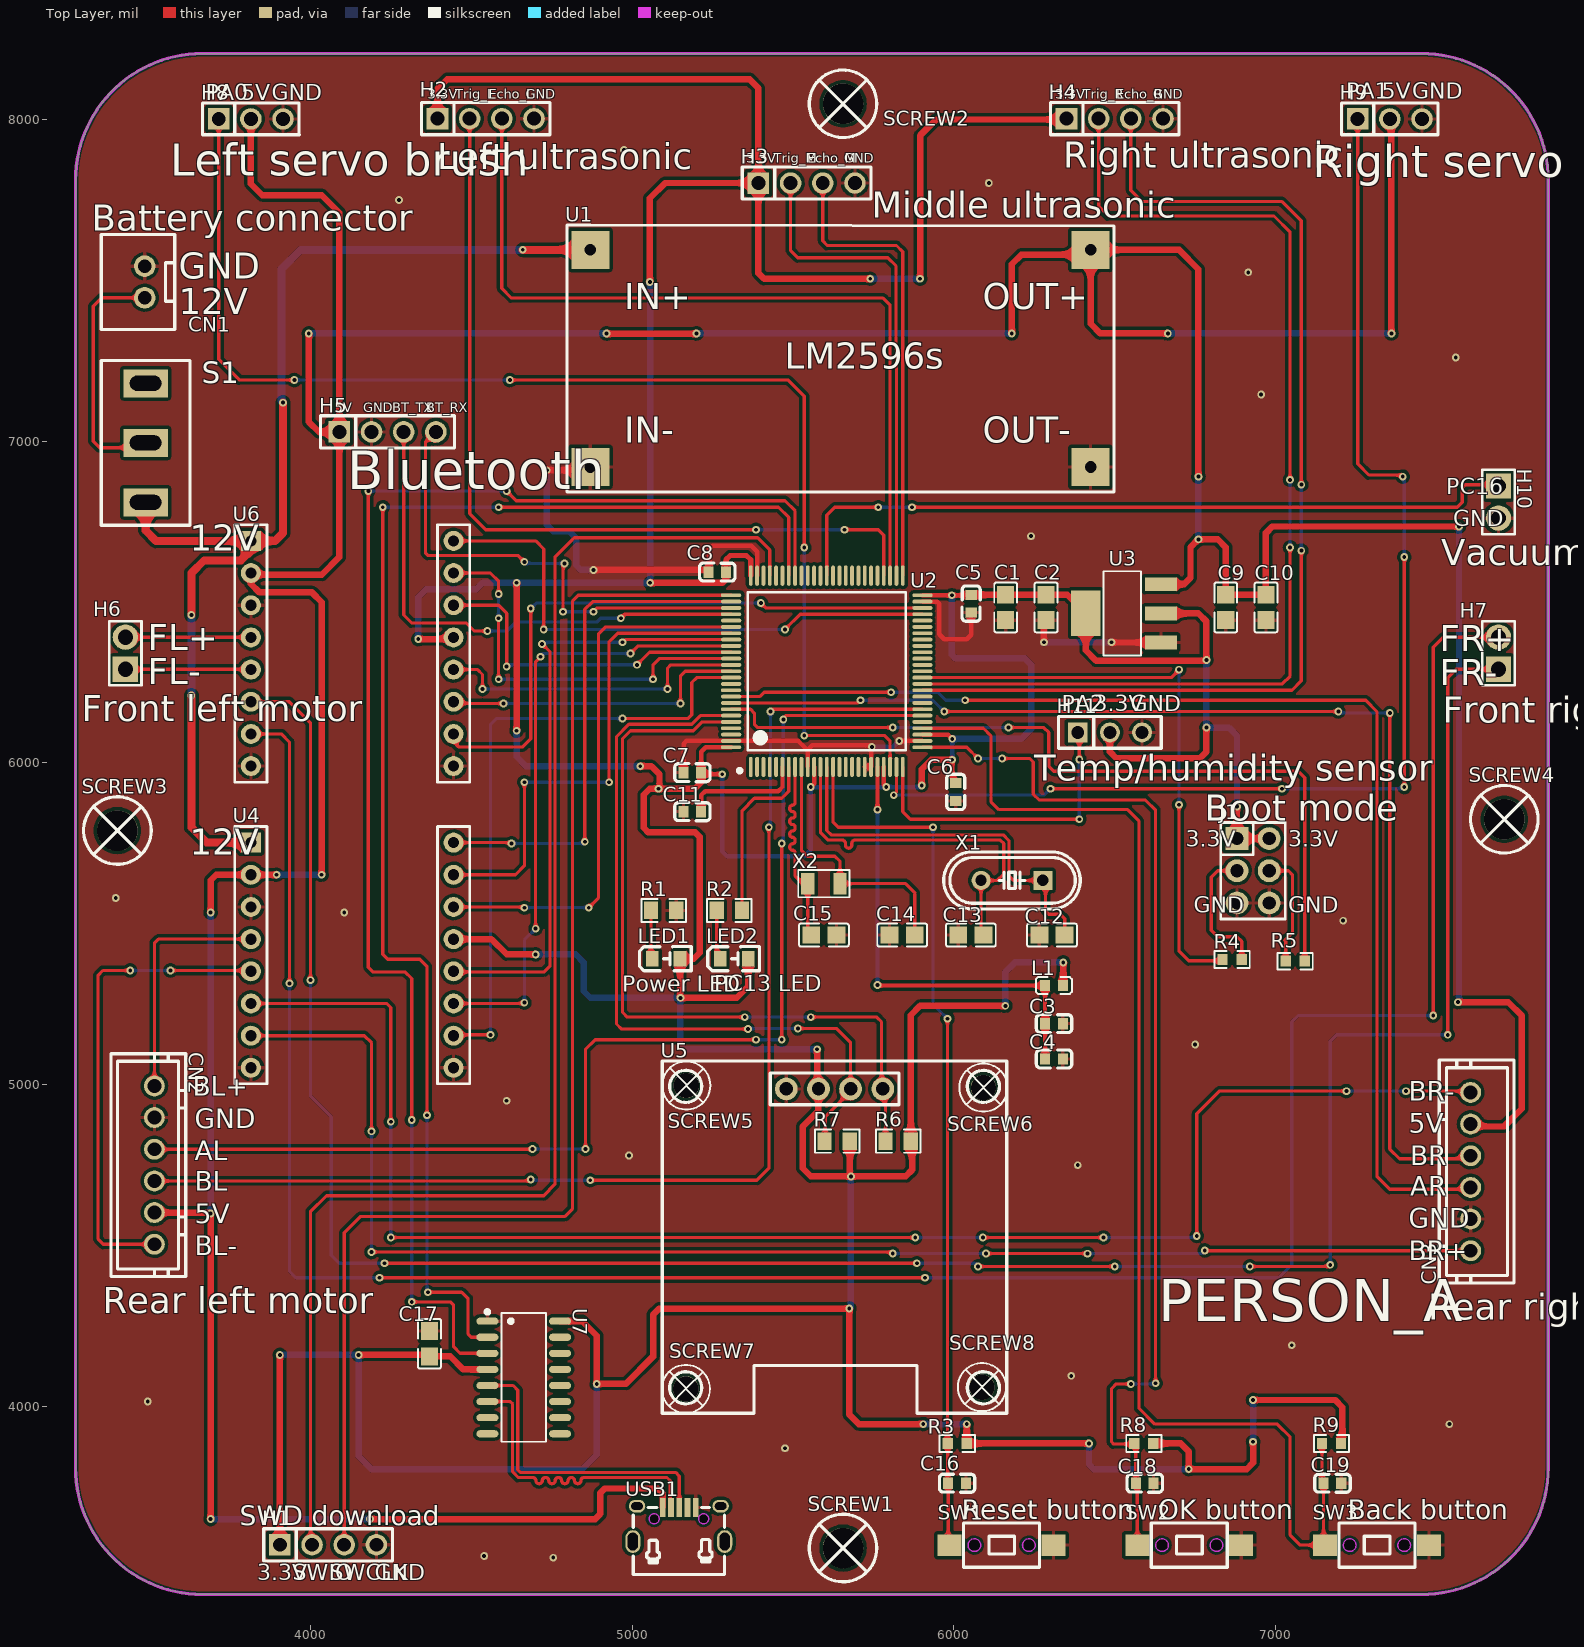
[diagram p0: Top Layer view]
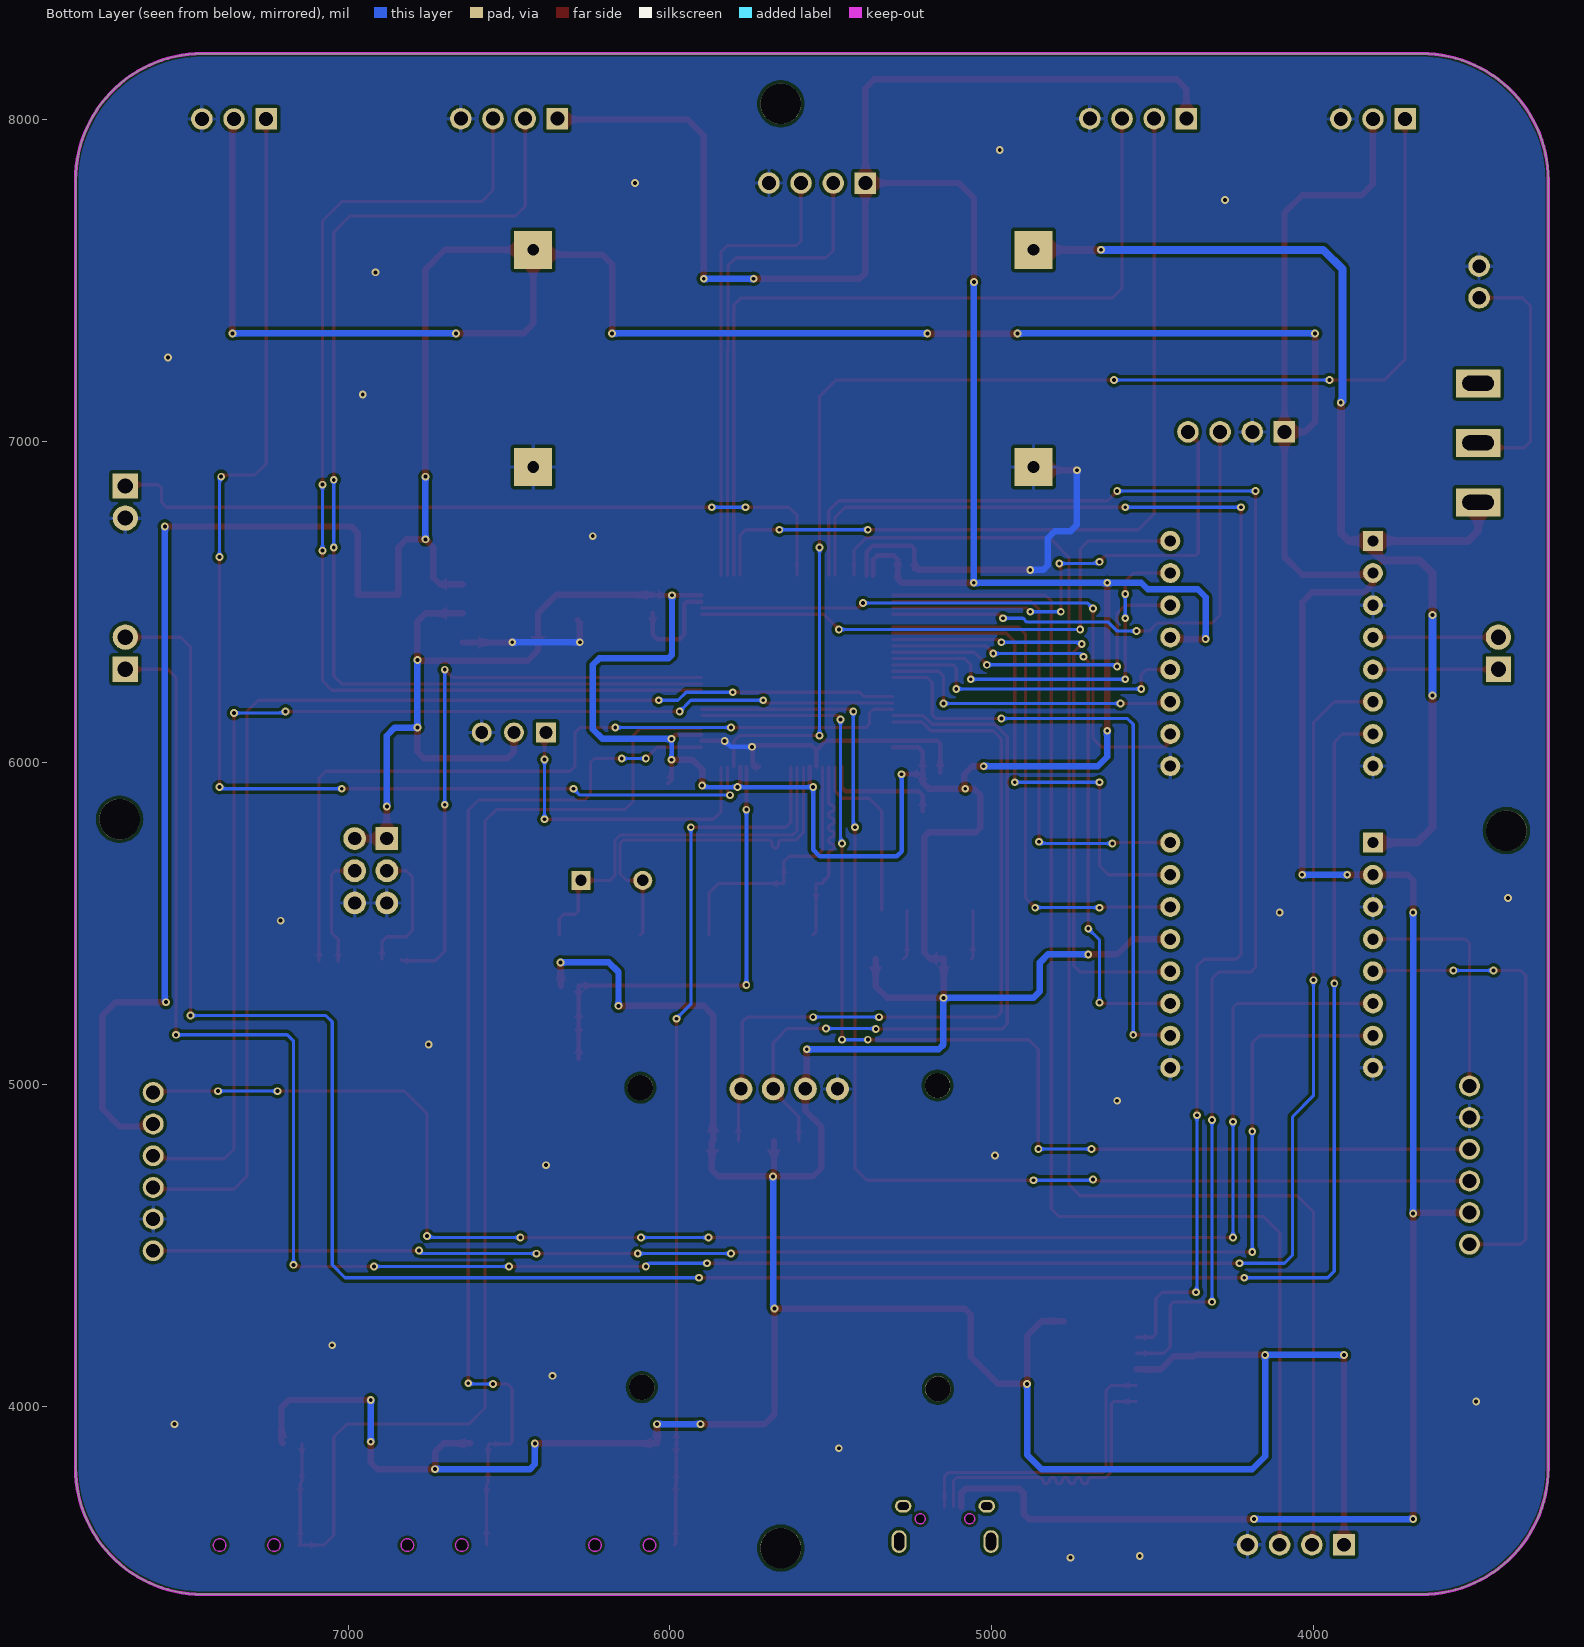
[diagram p1: Bottom Layer view, seen from below]
# Altium PCB MISC62445.pcbdoc (part 1 of 3)
Units mil, origin at the board's own origin, x right, y up, seen from the top; angles counter-clockwise.
Board outline 4577.56 x 4789.41 mil, 2 copper layers (Top Layer, Bottom Layer), stack 62.206 mil thick; 68 components, 65 nets, 307 pads, 204 vias.

## Layer stack, top to bottom
Top Solder Mask Layer: solder mask 0.394, Dk 3.3
Top Layer: signal copper 1.379
Dielectric1: surface 59.449, FR4, Dk 4.5
Bottom Layer: signal copper 1.378
Bottom Solder Mask Layer: solder mask 0.394, Dk 3.3

## Board outline
3663.7,8205 ccw(c3663.7,7811.3) 3270,7811.3 3270,3809.29 ccw(c3663.7,3809.29) 3663.7,3415.59 7453.86,3415.59 ccw(c7453.86,3809.29) 7847.56,3809.29 7847.56,7811.3 ccw(c7453.86,7811.3) 7453.86,8205

## Design rules (kind name [scope] priority, off if disabled: settings)
BoardOutlineClearance copperThickness2oz_1 [All] p2 off: genericclearance=7.99 ignorepadtopadclearanceinfootprint=FALSE except(0: Arc-SplitContinuation Track-SplitContinuation SMDPad-SplitContinuation THPad-SplitContinuation Via-SplitContinuation Fill-SplitContinuation Region-SplitContinuation Poly-SplitContinuation Text-SplitContinuation Hole-SplitContinuation; 5.98: Arc-CutoutEdge Track-CutoutEdge SMDPad-CutoutEdge THPad-CutoutEdge Via-CutoutEdge Text-CutoutEdge; 6.9: Hole-OutlineEdge Hole-CutoutEdge; 10: Poly-OutlineEdge Poly-CutoutEdge; 11.81: Arc-OutlineEdge Track-OutlineEdge SMDPad-OutlineEdge THPad-OutlineEdge Via-OutlineEdge Fill-OutlineEdge Region-OutlineEdge Text-OutlineEdge Fill-CutoutEdge Region-CutoutEdge)
BoardOutlineClearance Plane_innerPlane_1 [All] p4 off: genericclearance=4.02 ignorepadtopadclearanceinfootprint=FALSE except(0: Arc-SplitContinuation Track-SplitContinuation SMDPad-SplitContinuation THPad-SplitContinuation Via-SplitContinuation Fill-SplitContinuation Region-SplitContinuation Poly-SplitContinuation Text-SplitContinuation Hole-SplitContinuation; 5.98: Arc-CutoutEdge Track-CutoutEdge SMDPad-CutoutEdge THPad-CutoutEdge Via-CutoutEdge Text-CutoutEdge; 6.9: Hole-OutlineEdge Hole-CutoutEdge; 10: Poly-OutlineEdge Poly-CutoutEdge; 11.81: Arc-OutlineEdge Track-OutlineEdge SMDPad-OutlineEdge THPad-OutlineEdge Via-OutlineEdge Fill-OutlineEdge Region-OutlineEdge Text-OutlineEdge Fill-CutoutEdge Region-CutoutEdge)
BoardOutlineClearance Copper_copperRegion_1 [All] p6 off: genericclearance=4.02 ignorepadtopadclearanceinfootprint=FALSE except(0: Arc-SplitContinuation Track-SplitContinuation SMDPad-SplitContinuation THPad-SplitContinuation Via-SplitContinuation Fill-SplitContinuation Region-SplitContinuation Poly-SplitContinuation Text-SplitContinuation Hole-SplitContinuation; 5.98: Arc-CutoutEdge Track-CutoutEdge SMDPad-CutoutEdge THPad-CutoutEdge Via-CutoutEdge Text-CutoutEdge; 6.9: Hole-OutlineEdge Hole-CutoutEdge; 10: Poly-OutlineEdge Poly-CutoutEdge; 11.81: Arc-OutlineEdge Track-OutlineEdge SMDPad-OutlineEdge THPad-OutlineEdge Via-OutlineEdge Fill-OutlineEdge Region-OutlineEdge Text-OutlineEdge Fill-CutoutEdge Region-CutoutEdge)
BoardOutlineClearance copperThickness1oz_1 [All] p8: genericclearance=4.02 ignorepadtopadclearanceinfootprint=FALSE except(0: Arc-SplitContinuation Track-SplitContinuation SMDPad-SplitContinuation THPad-SplitContinuation Via-SplitContinuation Fill-SplitContinuation Region-SplitContinuation Poly-SplitContinuation Text-SplitContinuation Hole-SplitContinuation; 5.98: Arc-CutoutEdge Track-CutoutEdge SMDPad-CutoutEdge THPad-CutoutEdge Via-CutoutEdge Text-CutoutEdge; 6.9: Hole-OutlineEdge Hole-CutoutEdge; 10: Poly-OutlineEdge Poly-CutoutEdge; 11.81: Arc-OutlineEdge Track-OutlineEdge SMDPad-OutlineEdge THPad-OutlineEdge Via-OutlineEdge Fill-OutlineEdge Region-OutlineEdge Text-OutlineEdge Fill-CutoutEdge Region-CutoutEdge)
Clearance copperThickness2oz [All] p1 off: gap=7.99 ignorepadtopadclearanceinfootprint=FALSE except(5.98: SMDPad-Track SMDPad-SMDPad THPad-Track SMDPad-THPad THPad-THPad Track-Via SMDPad-Via THPad-Via Via-Via Fill-SMDPad Region-SMDPad Fill-THPad Region-THPad Fill-Via Region-Via Fill-Fill Fill-Region Region-Region Arc-Track Arc-SMDPad Arc-THPad Arc-Via Fill-Arc Region-Arc Arc-Arc Text-Track SMDPad-Text Text-THPad Text-Via Fill-Text Region-Text Arc-Text Text-Text; 6.9: Hole-Track Hole-SMDPad Hole-THPad Hole-Via Fill-Hole Region-Hole Hole-Arc Hole-Text; 10: Poly-Track Poly-SMDPad Poly-THPad Poly-Via Poly-Fill Poly-Region Poly-Poly Poly-Arc Poly-Text Poly-Hole; 11.81: Fill-Track Region-Track)
Clearance Plane_innerPlane [All] p3 off: gap=4.02 ignorepadtopadclearanceinfootprint=FALSE except(5.98: SMDPad-Track SMDPad-SMDPad THPad-Track SMDPad-THPad THPad-THPad Track-Via SMDPad-Via THPad-Via Via-Via Fill-SMDPad Region-SMDPad Fill-THPad Region-THPad Fill-Via Region-Via Fill-Fill Fill-Region Region-Region Arc-Track Arc-SMDPad Arc-THPad Arc-Via Fill-Arc Region-Arc Arc-Arc Text-Track SMDPad-Text Text-THPad Text-Via Fill-Text Region-Text Arc-Text Text-Text; 6.9: Hole-Track Hole-SMDPad Hole-THPad Hole-Via Fill-Hole Region-Hole Hole-Arc Hole-Text; 10: Poly-Track Poly-SMDPad Poly-THPad Poly-Via Poly-Fill Poly-Region Poly-Poly Poly-Arc Poly-Text Poly-Hole; 11.81: Fill-Track Region-Track)
Clearance Copper_copperRegion [All] p5 off: gap=4.02 ignorepadtopadclearanceinfootprint=FALSE except(5.98: SMDPad-Track SMDPad-SMDPad THPad-Track SMDPad-THPad THPad-THPad Track-Via SMDPad-Via THPad-Via Via-Via Fill-SMDPad Region-SMDPad Fill-THPad Region-THPad Fill-Via Region-Via Fill-Fill Fill-Region Region-Region Arc-Track Arc-SMDPad Arc-THPad Arc-Via Fill-Arc Region-Arc Arc-Arc Text-Track SMDPad-Text Text-THPad Text-Via Fill-Text Region-Text Arc-Text Text-Text; 6.9: Hole-Track Hole-SMDPad Hole-THPad Hole-Via Fill-Hole Region-Hole Hole-Arc Hole-Text; 10: Poly-Track Poly-SMDPad Poly-THPad Poly-Via Poly-Fill Poly-Region Poly-Poly Poly-Arc Poly-Text Poly-Hole; 11.81: Fill-Track Region-Track)
Clearance copperThickness1oz [All] p7: gap=4.02 ignorepadtopadclearanceinfootprint=FALSE except(5.98: SMDPad-Track SMDPad-SMDPad THPad-Track SMDPad-THPad THPad-THPad Track-Via SMDPad-Via THPad-Via Via-Via Fill-SMDPad Region-SMDPad Fill-THPad Region-THPad Fill-Via Region-Via Fill-Fill Fill-Region Region-Region Arc-Track Arc-SMDPad Arc-THPad Arc-Via Fill-Arc Region-Arc Arc-Arc Text-Track SMDPad-Text Text-THPad Text-Via Fill-Text Region-Text Arc-Text Text-Text; 6.9: Hole-Track Hole-SMDPad Hole-THPad Hole-Via Fill-Hole Region-Hole Hole-Arc Hole-Text; 10: Poly-Track Poly-SMDPad Poly-THPad Poly-Via Poly-Fill Poly-Region Poly-Poly Poly-Arc Poly-Text Poly-Hole; 11.81: Fill-Track Region-Track)
DiffPairsRouting differentialPair [All] p1: maxlimit=6 minlimit=6 mostfreqgap=6 toplayer_minwidth=5 toplayer_prefwidth=10 toplayer_maxwidth=100 toplayer_mingap=6 toplayer_prefgap=6 toplayer_maxgap=6 bottomlayer_minwidth=5 bottomlayer_prefwidth=10 bottomlayer_maxwidth=100 bottomlayer_mingap=6 bottomlayer_prefgap=6 bottomlayer_maxgap=6 maxuncoupledlength=10
HoleToHoleClearance otherClearance [All] p1: gap=11.81 allowstackedmicrovias=TRUE
Length netLength [All] p1: minlimit=0 maxlimit=0
PasteMaskExpansion pasteMaskExpansion [All] p1: expansion=0
PlaneConnect innerPlane [All] p1: planeconnectstyle=Relief reliefexpansion=20 reliefentries=4 reliefconductorwidth=10 reliefairgap=10
PolygonConnect copperRegion [All] p1: connectstyle=Relief reliefconductorwidth=10 reliefentries=4 polygonreliefangle="90 Angle" airgapwidth=10 via.connectstyle=Relief via.reliefconductorwidth=10 via.reliefentries=4 via.polygonreliefangle="90 Angle" via.airgapwidth=10
RoutingVias viaSize [All] p1: holewidth=12.01 width=24.02 viastyle="Through Hole" minholewidth=11.81 minwidth=19.68 maxholewidth=248.03 maxwidth=393.7
SolderMaskExpansion solderMaskExpansion [IsVia] p1: expansion=-1000 istentingtop=TRUE
SolderMaskExpansion solderMaskExpansion [All] p2: expansion=2 istentingtop=FALSE
Width copperThickness2oz_2 [All] p1 off: maxlimit=100 minlimit=8 preferedwidth=10
Width copperThickness1oz_2 [All] p2: maxlimit=100 minlimit=5 preferedwidth=10

## Components (designator, comment, footprint, x,y, rotation, side; value= is the part's Value field where it differs from the comment)
C1 "10uF" C0805 6161.05,6483.27 r90 top
C2 "100nF" C0805 6286.5,6483.27 r90 top
C3 "100nF" C0603 6311.09,5190 r180 top
C4 "10uF" C0603 6311.09,5080 r180 top
C5 "100nF" C0603 6053.62,6495.08 r270 top
C6 "100nF" C0603 6005.59,5909.77 r270 top
C7 "100nF" C0603 5187,5970 r180 top
C8 "100nF" C0603 5264.45,6593.37 r180 top
C9 "10uF" C0805 6845,6483.27 r90 top
C10 "100nF" C0805 6970,6483.27 r90 top
C11 "100nF" C0603 5187,5848.75 r180 top
C12 "20pF" C0805 6305,5465 r0 top
C13 "20pF" C0805 6052.95,5465 r0 top
C14 "20pF" C0805 5839.16,5465 r0 top
C15 "20pF" C0805 5596.06,5465 r180 top
C16 "1uF" C0603 6009.78,3761.54 r180 top
C17 "100pF" C0805 4370,4195 r270 top
C18 "1uF" C0603 6593.15,3761.54 r180 top
C19 "1uF" C0603 7176.51,3761.54 r180 top
CN1 "XH2.54*2P_THT" CONN-TH_2P-P2.50-XH2.54-2P 3485,7495 r270 top
CN2 "Rear left motor" CONN-TH_XH2.54-6P 3515,4750.06 r270 top
CN3 "Rear right motor" CONN-TH_XH2.54-6P 7606.27,4730 r90 top
H1 "SWD" HDR-TH_4P-P2.54-V-M 4055,3570 r0 top
H2 "Ultrasonic left" HDR-TH_4P-P2.54-V-M 4544.98,8002.56 r0 top
H3 "Ultrasonic middle" HDR-TH_4P-P2.54-V-M 5542.5,7802.56 r0 top
H4 "Ultrasonic right" HDR-TH_4P-P2.54-V-M 6500.02,8002.56 r0 top
H5 "2.54-1*4P female" HDR-TH_4P-P2.54-V-F 4240,7029.1 r0 top
H6 "Front left motor" HDR-TH_2P-P2.54-V-M 3425,6340.99 r90 top
H7 "Front right motor" HDR-TH_2P-P2.54-V-M 7692.83,6340.99 r90 top
H8 "PZ254V-11-03P" HDR-TH_3P-P2.54-V-M 3815,8001.77 r0 top
H9 "PZ254V-11-03P" HDR-TH_3P-P2.54-V-M 7355,8001.77 r0 top
H10 "PZ254V-11-02P" HDR-TH_2P-P2.54-V-M 7692.83,6810.94 r270 top
H11 "PM254V-11-03-H85" HDR-TH_3P-P2.54-V-F 6485,6095 r0 top
J1 "2.54-2*3P male pin" HDR-TH_6P-P2.54-V-M-R2-C3-S2.54-1 6930,5665 r270 top
L1 "10uH" L0603 6311.1,5307.86 r0 top
LED1 "NCD0805R1" LED0805-RD_RED 5105.63,5391.4 r0 top
LED2 "NCD0805R1" LED0805-RD_RED 5317.56,5391.41 r0 top
R1 "680Ω" R0805 5097.82,5541.6 r0 top
R2 "680Ω" R0805 5302.22,5541.61 r0 top
R3 "10kΩ" R0603 6010.47,3885 r0 top
R4 "10kΩ" R0603 6865,5388.95 r0 top
R5 "10kΩ" R0603 7060.94,5383.95 r0 top
R6 "4.7kΩ" R0805 5826.69,4824.66 r180 top
R7 "4.7kΩ" R0805 5637.34,4824.66 r180 top
R8 "10kΩ" R0603 6590.34,3885 r0 top
R9 "10kΩ" R0603 7173.71,3885 r0 top
S1 "ss12d10 switch" SS12D10 3487.96,6810 r90 top
SCREW1 "" M3螺丝 5655.5,3559.9 r0 top
SCREW2 "" M3螺丝 5655.5,8048.74 r0 top
SCREW3 "" M3螺丝 3400,5790 r0 top
SCREW4 "" M3螺丝 7710.83,5825 r0 top
SCREW5 "" M2螺丝 5168.32,4997.44 r0 top
SCREW6 "" M2螺丝 6091.96,4990.92 r0 top
SCREW7 "" M2螺丝 5167.09,4054.37 r0 top
SCREW8 "" M2螺丝 6087.28,4060 r0 top
SW1 "1TS002C-2300-4300-CT" SW-SMD_L6.0-W3.5-LS8.0-EH 6148.27,3568.9 r0 top
SW2 "1TS002C-2300-4300-CT" SW-SMD_L6.0-W3.5-LS8.0-EH 6731.63,3568.9 r0 top
SW3 "1TS002C-2300-4300-CT" SW-SMD_L6.0-W3.5-LS8.0-EH 7315,3568.9 r0 top
U1 "LM2596S buck module" LM2596S 4870,7595 r0 top
U2 "STM32F103VET6" LQFP-100_L14.0-W14.0-P0.50-LS16.0-BL 5605,6285 r0 top
U3 "AMS1117-3.3" SOT-223-3_L6.5-W3.4-P2.30-LS7.0-BR 6527.05,6465 r0 top
U4 "TB6612 module" TB6612-2X8 3815,5752.44 r0 top
U5 "HS96L03W2C03" OLED-TH_L27.8-W27.2-P2.54_C9900033791 5629.11,4986.98 r0 top
U6 "TB6612 module" TB6612-2X8 3815,6690.26 r0 top
U7 "CH340C" SOP-16_L10.0-W3.9-P1.27-LS6.0-BL 4663.1,4090 r270 top
USB1 "USB Android female socket" MICRO-USB-SMD_MICRO-USB-A8 5145,3635 r0 top
X1 "-" HC-49US_L11.5-W4.5-P4.88 6180.51,5635 r180 top
X2 "32.768kHz" OSC-SMD_L3.2-W1.5 5596.06,5625 r180 top

## Footprints (in the part's own frame and the unit in brackets; to place one, negate y for a bottom-side part, rotate by r counter-clockwise, add the part's x,y. Pads: shape width x height; smd on the part's side, far side on the other; paste and mask are expansions set on the pad)
C0603 [mm]
  rect 0.8x0.9 smd paste+0 mask+0.051: 1(-0.7,0) 2(0.7,0)
  silkscreen extent -1.41,-0.71 1.39,0.72
C0805 [mm]
  rect 1.41x1.35 smd paste-100 mask+0.051: 1(-1,0) 2(1,0)
  silkscreen extent -1.96,-0.9 1.96,0.9
CONN-TH_2P-P2.50-XH2.54-2P [mm]
  round 1.7 hole 1.05 paste+0 mask+0.05: 1(1.25,0) 2(-1.25,0)
  silkscreen extent -3.75,-3.42 3.75,2.37
CONN-TH_XH2.54-6P [mm]
  round 1.65 hole 1.1 paste+0 mask+0.05: 1(-6.25,0) 2(-3.75,0) 3(-1.25,0) 4(1.25,0) 5(3.75,0) 6(6.25,0)
  silkscreen extent -8.8,-3.43 8.8,2.47
HC-49US_L11.5-W4.5-P4.88 [mm]
  rect 1.5x1.5 hole 0.9: 1(-2.44,0)
  round 1.5 hole 0.9: 2(2.44,0)
  silkscreen extent -5.39,-2.25 5.39,2.25
HDR-TH_2P-P2.54-V-M [mm]
  rect 2x2 hole 1.2: 1(-1.27,0)
  round 2 hole 1.2: 2(1.27,0)
  silkscreen extent -2.54,-1.27 2.54,1.27
HDR-TH_3P-P2.54-V-F [mil]
  rect 62x62 hole 40.16: 1(-100,0)
  round 62 hole 40.16: 2(0,0) 3(100,0)
  silkscreen extent -160,-49 160,49
HDR-TH_3P-P2.54-V-M [mm]
  rect 1.7x1.7 hole 1.1: 1(-2.54,0)
  round 1.7 hole 1.1: 2(0,0) 3(2.54,0)
  silkscreen extent -3.81,-1.25 3.81,1.25
HDR-TH_4P-P2.54-V-F [mm]
  rect 1.7x1.7 hole 1.1: 1(-3.81,0)
  round 1.7 hole 1.1: 2(-1.27,0) 3(1.27,0) 4(3.81,0)
  silkscreen extent -5.29,-1.27 5.29,1.27
HDR-TH_4P-P2.54-V-M [mm]
  rect 1.7x1.7 hole 1.1: 1(-3.81,0)
  round 1.7 hole 1.1: 2(-1.27,0) 3(1.27,0) 4(3.81,0)
  silkscreen extent -5.08,-1.27 5.08,1.27
HDR-TH_6P-P2.54-V-M-R2-C3-S2.54-1 [mm]
  rect 1.8x1.8 hole 1.05 paste+0 mask+0.051: 1(-2.54,-1.27)
  round 1.8 hole 1.05 paste+0 mask+0.051: 2(-2.54,1.27) 3(0,-1.27) 4(0,1.27) 5(2.54,-1.27) 6(2.54,1.27)
  silkscreen extent -3.81,-2.54 3.81,2.54
L0603 [mm]
  rect 0.8x0.864 smd paste-100 mask+0.051: 1(-0.7,0) 2(0.7,0)
  silkscreen extent -1.42,-0.65 1.41,0.67
LED0805-RD_RED [mm]
  rect 1x1.25 smd: 1(-1.1,0) 2(1.1,0)
  silkscreen extent -2.1,-0.95 1.98,0.96
LM2596S [mm]
  rect 3x3 hole 0.914 paste+0 mask+0.102: 1(0,0) 2(0,-17.145) 3(39.497,-17.145) 4(39.497,0)
  silkscreen extent -1.84,-19.11 41.34,1.97
LQFP-100_L14.0-W14.0-P0.50-LS16.0-BL [mm]
  oval 0.3x1.6 smd: 1(-6,-7.55) 2(-5.5,-7.55) 3(-5,-7.55) 4(-4.5,-7.55) 5(-4,-7.55) 6(-3.5,-7.55) 7(-3,-7.55) 8(-2.5,-7.55) 9(-2,-7.55) 10(-1.5,-7.55) 11(-1,-7.55) 12(-0.5,-7.55) 13(0,-7.55) 14(0.5,-7.55) 15(1,-7.55) 16(1.5,-7.55) 17(2,-7.55) 18(2.5,-7.55) 19(3,-7.55) 20(3.5,-7.55) 21(4,-7.55) 22(4.5,-7.55) 23(5,-7.55) 24(5.5,-7.55) 25(6,-7.55) 51(6,7.55) 52(5.5,7.55) 53(5,7.55) 54(4.5,7.55) 55(4,7.55) 56(3.5,7.55) 57(3,7.55) 58(2.5,7.55) 59(2,7.55) 60(1.5,7.55) 61(1,7.55) 62(0.5,7.55) 63(0,7.55) 64(-0.5,7.55) 65(-1,7.55) 66(-1.5,7.55) 67(-2,7.55) 68(-2.5,7.55) 69(-3,7.55) 70(-3.5,7.55) 71(-4,7.55) 72(-4.5,7.55) 73(-5,7.55) 74(-5.5,7.55) 75(-6,7.55)
  oval 1.6x0.3 smd: 26(7.55,-6) 27(7.55,-5.5) 28(7.55,-5) 29(7.55,-4.5) 30(7.55,-4) 31(7.55,-3.5) 32(7.55,-3) 33(7.55,-2.5) 34(7.55,-2) 35(7.55,-1.5) 36(7.55,-1) 37(7.55,-0.5) 38(7.55,0) 39(7.55,0.5) 40(7.55,1) 41(7.55,1.5) 42(7.55,2) 43(7.55,2.5) 44(7.55,3) 45(7.55,3.5) 46(7.55,4) 47(7.55,4.5) 48(7.55,5) 49(7.55,5.5) 50(7.55,6) 76(-7.55,6) 77(-7.55,5.5) 78(-7.55,5) 79(-7.55,4.5) 80(-7.55,4) 81(-7.55,3.5) 82(-7.55,3) 83(-7.55,2.5) 84(-7.55,2) 85(-7.55,1.5) 86(-7.55,1) 87(-7.55,0.5) 88(-7.55,0) 89(-7.55,-0.5) 90(-7.55,-1) 91(-7.55,-1.5) 92(-7.55,-2) 93(-7.55,-2.5) 94(-7.55,-3) 95(-7.55,-3.5) 96(-7.55,-4) 97(-7.55,-4.5) 98(-7.55,-5) 99(-7.55,-5.5) 100(-7.55,-6)
  silkscreen extent -7.03,-8 6.25,6.25
M2螺丝 [mm]
  round 2 hole 2: 1(0,0)
  silkscreen extent -1.9,-1.9 1.9,1.9
M3螺丝 [mil]
  round 126 hole 126 paste+0 mask+4: 1(0,0)
  silkscreen extent -105,-105 105,105
MICRO-USB-SMD_MICRO-USB-A8 [mm]
  rect 0.45x1.5 smd paste-100 mask+0.051: 1(-1.265,1.3) 2(-0.615,1.3) 3(0.036,1.3) 4(0.686,1.3) 5(1.336,1.3)
  oval 1.3x1 hole 0.6 slot 0.9 at 0 deg copper offset 0.001,0.001: 6(3.304,1.399)
  oval 1.3x1 hole 0.6 slot 0.9 at 0 deg copper offset 0.001,-0.001: 7(-3.295,1.4)
  oval 1.2x1.8 hole 0.8 slot 1.4 at 90 deg copper offset -0.001,0: 8(3.625,-1.4)
  oval 1.2x1.8 hole 0.8 slot 1.4 at 90 deg: 9(-3.625,-1.4)
  Board Outline Layer circle w0.003: c1.956,0.401 r0.4
  Board Outline Layer circle w0.003: c-1.946,0.401 r0.4
  Board Outline Layer region: 2.356,0.401 2.316,0.228 2.205,0.089 2.045,0.011 1.867,0.011 1.706,0.089 1.595,0.228 1.556,0.401 1.556,0.401 1.595,0.575 1.706,0.714 1.867,0.791 2.045,0.791 2.205,0.714 2.316,0.575 2.356,0.401
  Board Outline Layer region: 2.356,0.401 2.346,0.312 2.316,0.228 2.269,0.152 2.205,0.089 2.129,0.041 2.045,0.011 1.956,0.001 1.867,0.011 1.782,0.041 1.706,0.089 1.643,0.152 1.595,0.228 1.566,0.312 1.556,0.401 1.566,0.49 1.595,0.575 1.643,0.651 1.706,0.714 1.782,0.762 1.867,0.791 1.956,0.801 2.045,0.791 2.129,0.762 2.205,0.714 2.269,0.651 2.316,0.575 2.346,0.49
  Board Outline Layer region: -1.546,0.401 -1.585,0.228 -1.696,0.089 -1.857,0.011 -2.035,0.011 -2.195,0.089 -2.306,0.228 -2.346,0.401 -2.346,0.401 -2.306,0.575 -2.195,0.714 -2.035,0.791 -1.857,0.791 -1.696,0.714 -1.585,0.575 -1.546,0.401
  Board Outline Layer region: -1.546,0.401 -1.556,0.312 -1.585,0.228 -1.633,0.152 -1.696,0.089 -1.772,0.041 -1.857,0.011 -1.946,0.001 -2.035,0.011 -2.119,0.041 -2.195,0.089 -2.258,0.152 -2.306,0.228 -2.336,0.312 -2.346,0.401 -2.336,0.49 -2.306,0.575 -2.258,0.651 -2.195,0.714 -2.119,0.762 -2.035,0.791 -1.946,0.801 -1.857,0.791 -1.772,0.762 -1.696,0.714 -1.633,0.651 -1.585,0.575 -1.556,0.49
  Multi-Layer board cut-out: 2.356,0.401 2.316,0.228 2.205,0.089 2.045,0.011 1.867,0.011 1.706,0.089 1.595,0.228 1.556,0.401 1.556,0.401 1.595,0.575 1.706,0.714 1.867,0.791 2.045,0.791 2.205,0.714 2.316,0.575 2.356,0.401
  Multi-Layer board cut-out: -1.546,0.401 -1.585,0.228 -1.696,0.089 -1.857,0.011 -2.035,0.011 -2.195,0.089 -2.306,0.228 -2.346,0.401 -2.346,0.401 -2.306,0.575 -2.195,0.714 -2.035,0.791 -1.857,0.791 -1.696,0.714 -1.585,0.575 -1.546,0.401
  silkscreen extent -3.59,-4 3.61,1.3
OLED-TH_L27.8-W27.2-P2.54_C9900033791 [mm]
  round 1.8 hole 1.05 paste+0 mask+0.05: 1(-3.81,0) 2(-1.27,0) 3(1.27,0) 4(3.81,0)
  silkscreen extent -13.6,-25.6 13.6,2.2
OSC-SMD_L3.2-W1.5 [mm]
  rect 1.05x1.7 smd: 1(-1.275,0) 2(1.275,0)
  silkscreen extent -2.03,-1.08 2.03,1.08
R0603 [mil]
  rect 31.75x34.02 smd paste-3937.01 mask+2: 1(-29.66,0) 2(29.66,0)
  silkscreen extent -55,-26 55,26
R0805 [mm]
  rect 1.133x1.377 smd paste-100 mask+0.051: 1(-1,0) 2(1,0)
  silkscreen extent -1.76,-0.92 1.76,0.92
SOP-16_L10.0-W3.9-P1.27-LS6.0-BL [mm]
  oval 0.56x1.745 smd: 1(-4.445,-2.872) 2(-3.175,-2.872) 3(-1.905,-2.872) 4(-0.635,-2.872) 5(0.635,-2.872) 6(1.905,-2.872) 7(3.175,-2.872) 8(4.445,-2.872) 9(4.445,2.872) 10(3.175,2.872) 11(1.905,2.872) 12(0.635,2.872) 13(-0.635,2.872) 14(-1.905,2.872) 15(-3.175,2.872) 16(-4.445,2.872)
  silkscreen extent -5.33,-3.02 5.08,1.77
SOT-223-3_L6.5-W3.4-P2.30-LS7.0-BR [mm]
  rect 2.5x1.1 smd: 1(2.97,-2.3) 2(2.97,0) 3(2.97,2.3)
  rect 2.34x3.6 smd: 4(-2.97,0)
  silkscreen extent -1.57,-3.33 1.37,3.33
SS12D10 [mil]
  rect 86.6x137.8 hole 47.2 slot 98.4 at 90 deg paste+0 mask+4: 1(0,0) 2(185,0) 3(370,0)
  silkscreen extent -71,-138 441,138
SW-SMD_L6.0-W3.5-LS8.0-EH [mm]
  rect 1.9x1.7 smd: 1(-4.1,0) 2(4.1,0)
  Board Outline Layer circle w0.003: c-2.15,0 r0.5
  Board Outline Layer circle w0.003: c2.15,0 r0.5
  Board Outline Layer region: -1.65,0 -1.7,-0.217 -1.838,-0.391 -2.039,-0.487 -2.261,-0.487 -2.462,-0.391 -2.601,-0.217 -2.65,0 -2.65,0 -2.601,0.217 -2.462,0.391 -2.261,0.487 -2.039,0.487 -1.838,0.391 -1.7,0.217 -1.65,0
  Board Outline Layer region: -1.65,0 -1.66,-0.098 -1.688,-0.191 -1.734,-0.278 -1.797,-0.354 -1.872,-0.416 -1.959,-0.462 -2.053,-0.49 -2.15,-0.5 -2.248,-0.49 -2.341,-0.462 -2.428,-0.416 -2.504,-0.354 -2.566,-0.278 -2.612,-0.191 -2.641,-0.098 -2.65,0 -2.641,0.098 -2.612,0.191 -2.566,0.278 -2.504,0.354 -2.428,0.416 -2.341,0.462 -2.248,0.49 -2.15,0.5 -2.053,0.49 -1.959,0.462 -1.872,0.416 -1.797,0.354 -1.734,0.278 -1.688,0.191 -1.66,0.098
  Board Outline Layer region: 2.65,0 2.601,-0.217 2.462,-0.391 2.261,-0.487 2.039,-0.487 1.838,-0.391 1.7,-0.217 1.65,0 1.65,0 1.7,0.217 1.838,0.391 2.039,0.487 2.261,0.487 2.462,0.391 2.601,0.217 2.65,0
  Board Outline Layer region: 2.65,0 2.641,-0.098 2.612,-0.191 2.566,-0.278 2.504,-0.354 2.428,-0.416 2.341,-0.462 2.248,-0.49 2.15,-0.5 2.053,-0.49 1.959,-0.462 1.872,-0.416 1.797,-0.354 1.734,-0.278 1.688,-0.191 1.66,-0.098 1.65,0 1.66,0.098 1.688,0.191 1.734,0.278 1.797,0.354 1.872,0.416 1.959,0.462 2.053,0.49 2.15,0.5 2.248,0.49 2.341,0.462 2.428,0.416 2.504,0.354 2.566,0.278 2.612,0.191 2.641,0.098
  Multi-Layer board cut-out: -1.65,0 -1.7,-0.217 -1.838,-0.391 -2.039,-0.487 -2.261,-0.487 -2.462,-0.391 -2.601,-0.217 -2.65,0 -2.65,0 -2.601,0.217 -2.462,0.391 -2.261,0.487 -2.039,0.487 -1.838,0.391 -1.7,0.217 -1.65,0
  Multi-Layer board cut-out: 2.65,0 2.601,-0.217 2.462,-0.391 2.261,-0.487 2.039,-0.487 1.838,-0.391 1.7,-0.217 1.65,0 1.65,0 1.7,0.217 1.838,0.391 2.039,0.487 2.261,0.487 2.462,0.391 2.601,0.217 2.65,0
  silkscreen extent -3,-1.75 3,1.75
TB6612-2X8 [mil]
  rect 62x62 hole 35: 1(0,0)
  round 62 hole 35: 2(0,-100) 3(0,-200) 4(0,-300) 5(0,-400) 6(0,-500) 7(0,-600) 8(0,-700) 9(629.92,-700) 10(629.92,-600) 11(629.92,-500) 12(629.92,-400) 13(629.92,-300) 14(629.92,-200) 15(629.92,-100) 16(629.92,0)
  silkscreen extent -50,-750 680,50

## Via types
v1: diameter 24.02, hole 12, Top Layer to Bottom Layer, 204 vias

## Nets (pads, with @x,y where several pads share a name; then routed paths per layer and width w, separated by ;. In a path a pad name is that pad's centre, name@x,y a point inside that pad or via, vN(x,y) a via of type N, cw(c..) or ccw(c..) an arc to the next point about the centre after c; other vN are vias at no path point)
$1N3398: C11.1 U2.6 | length 376.6
  Top Layer w13: C11.1@5214.56,5848.75 5214.56,5899.56 5227.2,5912.2 5454.2,5912.2 5467.2,5925.2 U2.6@5467.2,5987.76
$1N3770: CN1.1 S1.2 | length 768.1
  Top Layer w10: CN1.1@3485,7445.79 3350.79,7445.79 3325,7420 3325,7000 3345,6980 3472.96,6980 S1.2@3487.96,6995
$1N4671: J1.4 R5.1 | length 357
  Top Layer w10: J1.4@6980,5665 7040,5665 7052.07,5652.93 7052.07,5472.07 7028.45,5448.45 7031.28,5445.63 R5.1@7031.28,5383.95
$1N4675: J1.3 R4.2 | length 418.7
  Top Layer w10: J1.3@6880,5665 6820,5665 6800,5645 6800,5480 6820,5460 6880,5460 6894.66,5445.34 R4.2@6894.66,5388.95
$1N4927: LED2.1 R2.1 | length 154.9
  Top Layer w10: R2.1@5262.85,5541.61 5262.85,5402.81 LED2.1@5274.25,5391.41
$1N5007: LED1.1 R1.1 | length 151.8
  Top Layer w10: R1.1@5058.45,5541.6 5058.45,5395.28 LED1.1@5062.32,5391.41